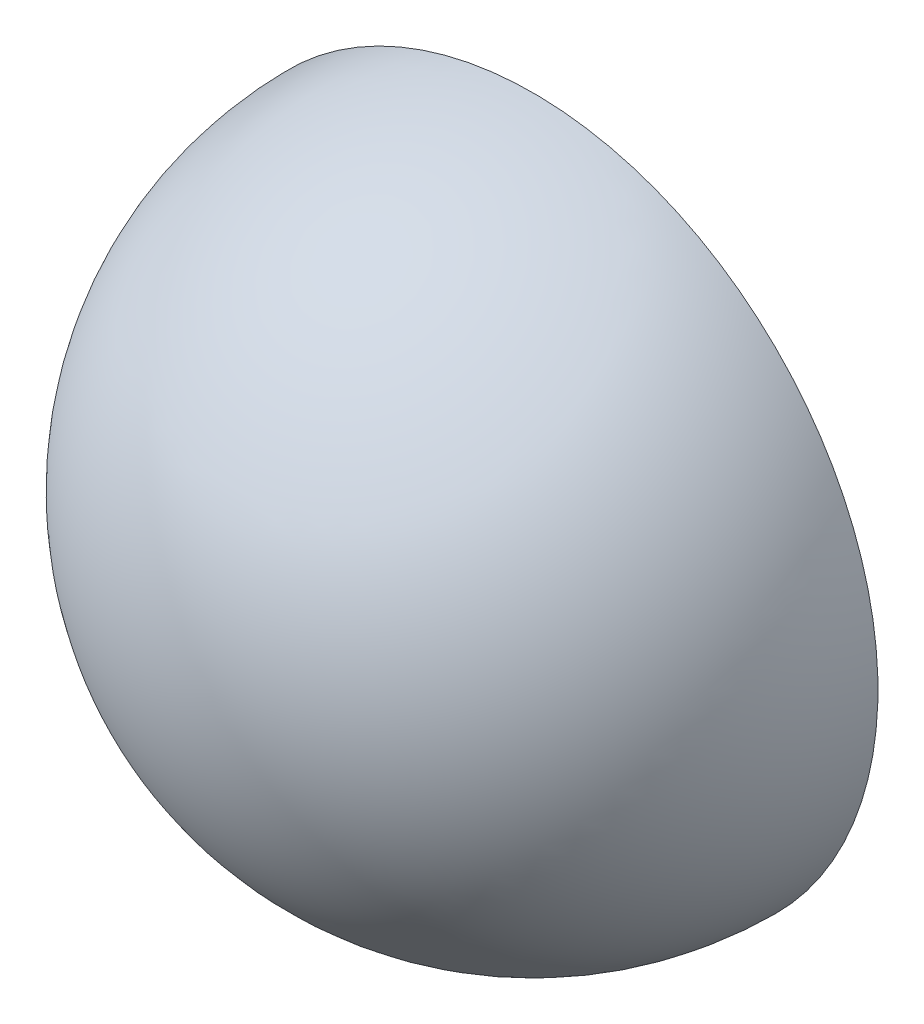
from build123d import *

# Parameters (mm, degrees)
REVOLVE_1_ANGLE = 180


with BuildPart() as part:
    # 草图1 → 旋转1 (revolve)
    with BuildSketch(Plane.XY):
        with BuildLine():
            Line((0, 70), (0, -70))
            ThreePointArc((0, -70), (70, 0), (0, 70))
        make_face()
    revolve(axis=Axis((0, 70, 0), (0, -1, 0)), revolution_arc=REVOLVE_1_ANGLE)


solid = part.part
